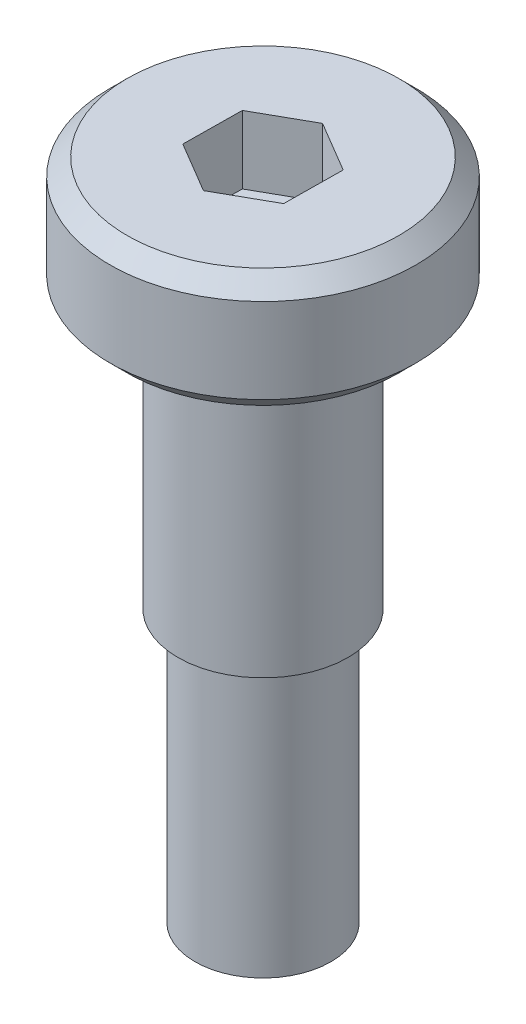
from build123d import *

# Parameters (mm, degrees)
CUT_EXTRUDE1_DEPTH = 2
CHAMFER1_SIZE      = 0.5


with BuildPart() as part:
    # Sketch1 → Revolve1 (revolve)
    with BuildSketch(Plane.XY, mode=Mode.PRIVATE) as revolve1_sk:
        Polygon((0, 0), (0, 19.5), (-4.5, 19.5), (-4.5, 16), (-2.5, 16), (-2.5, 8), (-2, 8), (-2, 0), align=None)
    revolve(revolve1_sk.sketch.rotate(Axis((0, 0, 0), (0, 1, 0)), 180), axis=Axis((0, 0, 0), (0, 1, 0)))

    # Sketch2 → Cut-Extrude1 (cut)
    with BuildSketch(Plane(origin=(0, 19.5, 0), x_dir=(1, 0, 0), z_dir=(0, 1, 0))):
        Polygon((1.50956506, 0.849242799), (0.019316692, 1.73194309), (-1.490248367, 0.882700291), (-1.50956506, -0.849242799), (-0.019316692, -1.73194309), (1.490248367, -0.882700291), align=None)
    extrude(amount=-CUT_EXTRUDE1_DEPTH, mode=Mode.SUBTRACT)

    # Chamfer1
    chamfer1_edges = [part.edges().sort_by_distance(p)[0] for p in [
        (-4.5, 16, 0),
        (-4.5, 19.5, 0),
    ]]
    chamfer(chamfer1_edges, length=CHAMFER1_SIZE)


solid = part.part
